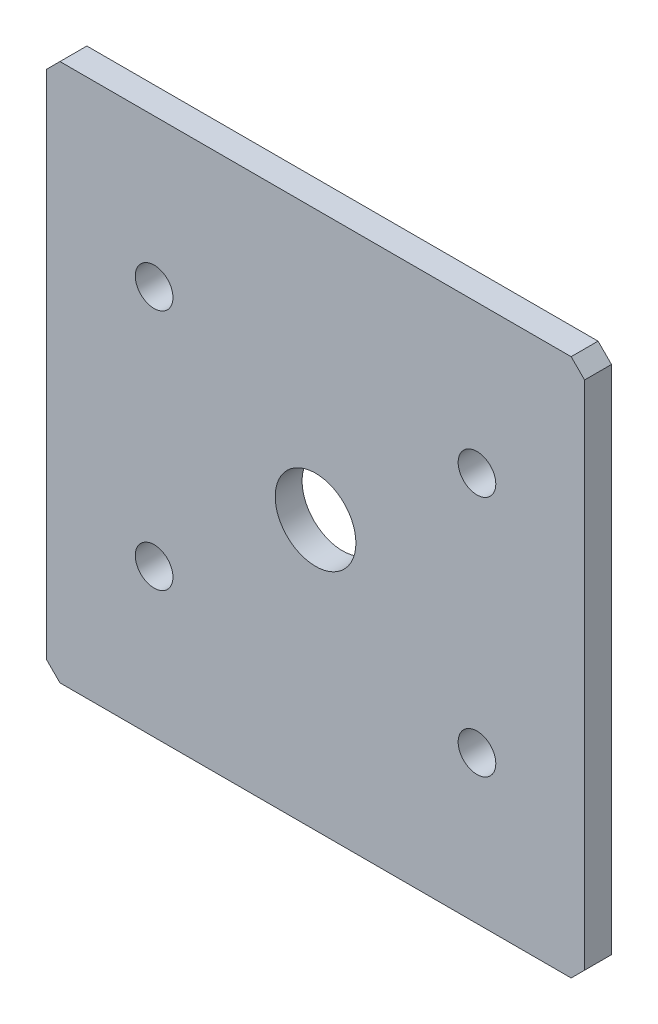
SolidWorks part; units mm, degrees
material "Q235-A "
ref_plane "前视基准面" through (0, 0, 0) normal (0, 0, 1) x (1, 0, 0)
ref_plane "上视基准面" through (0, 0, 0) normal (0, 1, 0) x (1, 0, 0)
ref_plane "右视基准面" through (0, 0, 0) normal (1, 0, 0) x (0, 0, -1)
sketch "草图1" plane through (0, 0, 0) normal (0, 0, 1) x (1, 0, 0)
  line L1 (0, 0) -> (200, 0)
  line L2 (0, 0) -> (0, -200)
  line L3 (0, -200) -> (200, -200)
  line L4 (200, 0) -> (200, -200)
  dimension "D1" = 200
  dimension "D2" = 200
extrude "凸台-拉伸1" add sketch "草图1" along normal blind 10
sketch "草图2" plane through (0, 0, 10) normal (0, 0, 1) x (1, 0, 0)
  line L0 (0, -100) -> (200, -100) construction
  line L1 (0, 0) -> (0, -200) construction
  line L2 (200, -200) -> (200, 0) construction
  line L3 (100, -100) -> (100, -200) construction
  line L4 (40, -55) -> (160, -55) construction
  line L5 (40, -55) -> (40, -145) construction
  line L6 (40, -145) -> (160, -145) construction
  line L7 (160, -55) -> (160, -145) construction
  line L8 (40, -55) -> (160, -145) construction
  line L9 (40, -145) -> (160, -55) construction
  line L10 (0, -200) -> (200, -200) construction
  circle A0 centre (40, -55) radius 7
  circle A1 centre (40, -145) radius 7
  circle A2 centre (160, -145) radius 7
  circle A3 centre (160, -55) radius 7
  circle A4 centre (100, -100) radius 15
  point P6 (100, -100)
  dimension "D4" = 14
  dimension "D3" = 30
  dimension "D1" = 120
  dimension "D2" = 90
extrude "切除-拉伸1" cut sketch "草图2" against normal through all
chamfer "倒角1" distance 5 angle 45 4 edges at (0, -200, 5) (200, -200, 5) (200, 0, 5) (0, 0, 5)
